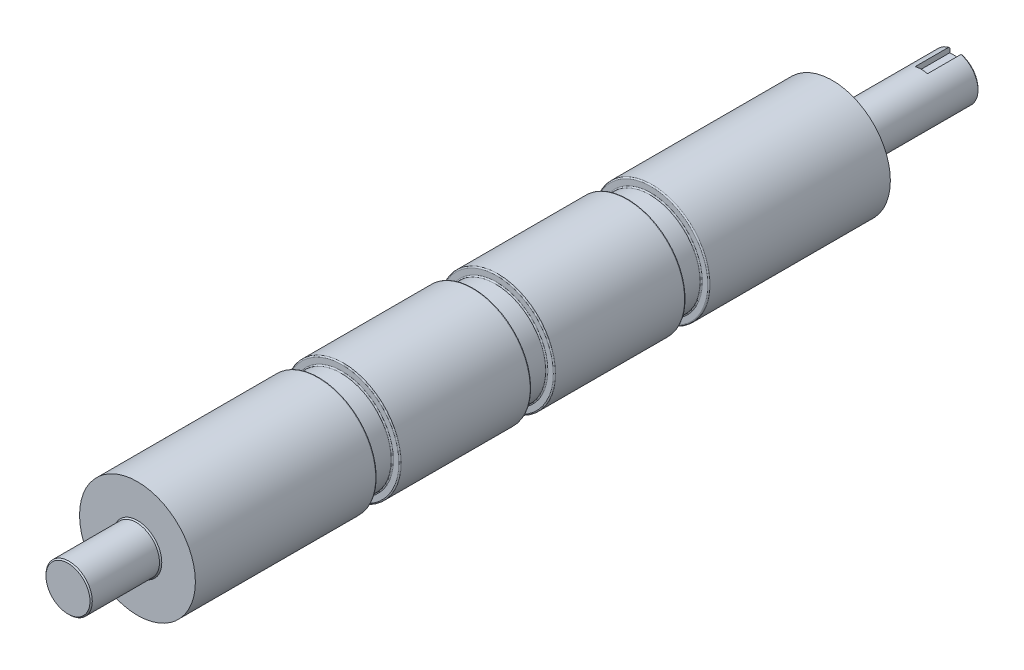
from build123d import *

# Parameters (mm, degrees)
SKETCH1_R                  = 150
BOSS_EXTRUDE1_DEPTH        = 1800
SKETCH2_W                  = 40
SKETCH2_H                  = 60
FILLET1_R                  = 3
LPATTERN1_COUNT            = 2
LPATTERN1_PITCH            = 400
FILLET1_OF_LPATTERN1_R     = 3
LPATTERN1_COL_COUNT        = 2
LPATTERN1_COL_PITCH        = 400
FILLET1_OF_LPATTERN1_COL_R = 3
SKETCH3_R                  = 60
BOSS_EXTRUDE2_DEPTH        = 180
CHAMFER1_SIZE              = 3
BOSS_EXTRUDE3_START        = 320
SKETCH4_R                  = 60
BOSS_EXTRUDE3_DEPTH        = 320
CHAMFER2_SIZE              = 3
SKETCH5_W                  = 32
SKETCH5_H                  = 32
CUT_EXTRUDE1_DEPTH         = 90


with BuildPart() as part:
    # Sketch1 → Boss-Extrude1 (new body)
    with BuildSketch(Plane.XY):
        Circle(SKETCH1_R)
    extrude(amount=BOSS_EXTRUDE1_DEPTH)

    # Sketch2 → Cut-Revolve1 (revolve, cut)
    with BuildSketch(Plane(origin=(0, 0, 0), x_dir=(1, 0, 0), z_dir=(0, 1, 0)), mode=Mode.PRIVATE) as cut_revolve1_sk:
        with Locations((150, -900)):
            Rectangle(SKETCH2_W, SKETCH2_H)
    cut_revolve1 = revolve(cut_revolve1_sk.sketch.rotate(Axis((0, 0, 0), (0, 0, 1)), 180), axis=Axis((0, 0, 0), (0, 0, 1)), mode=Mode.SUBTRACT)

    # Fillet1
    fillet1_edges = [part.edges().sort_by_distance(p)[0] for p in [
        (130, 0, 930),
        (-150, 0, 930),
        (130, 0, 870),
        (-150, 0, 870),
    ]]
    fillet(fillet1_edges, radius=FILLET1_R)

    # LPattern1: Cut-Revolve1 ×2
    with Locations(*[(0, 0, -i * LPATTERN1_PITCH) for i in range(1, LPATTERN1_COUNT)]):
        add(cut_revolve1, mode=Mode.SUBTRACT)

    # Fillet1 of LPattern1
    fillet1_of_lpattern1_edges = [part.edges().sort_by_distance(p)[0] for p in [
        (130, 0, 530),
        (-150, 0, 530),
        (130, 0, 470),
        (-150, 0, 470),
    ]]
    fillet(fillet1_of_lpattern1_edges, radius=FILLET1_OF_LPATTERN1_R)

    # LPattern1 col: Cut-Revolve1 ×2
    with Locations(*[(0, 0, i * LPATTERN1_COL_PITCH) for i in range(1, LPATTERN1_COL_COUNT)]):
        add(cut_revolve1, mode=Mode.SUBTRACT)

    # Fillet1 of LPattern1 col
    fillet1_of_lpattern1_col_edges = [part.edges().sort_by_distance(p)[0] for p in [
        (130, 0, 1330),
        (-150, 0, 1330),
        (130, 0, 1270),
        (-150, 0, 1270),
    ]]
    fillet(fillet1_of_lpattern1_col_edges, radius=FILLET1_OF_LPATTERN1_COL_R)

    # Sketch3 → Boss-Extrude2 (add)
    with BuildSketch(Plane.XY.offset(1800)):
        Circle(SKETCH3_R)
    extrude(amount=BOSS_EXTRUDE2_DEPTH)

    # Chamfer1
    chamfer1_edges = [part.edges().sort_by_distance(p)[0] for p in [
        (-60, 0, 1800),
        (-60, 0, 1980),
    ]]
    chamfer(chamfer1_edges, length=CHAMFER1_SIZE)

    # Sketch4 → Boss-Extrude3 (add)
    with BuildSketch(Plane(origin=(0, 0, 0), x_dir=(-1, 0, 0), z_dir=(0, 0, -1)).offset(BOSS_EXTRUDE3_START)):
        with Locations(Location((0, 0, 0), (0, 0, 180))):
            Circle(SKETCH4_R)
    extrude(amount=-BOSS_EXTRUDE3_DEPTH)

    # Chamfer2
    chamfer2_edges = [part.edges().sort_by_distance(p)[0] for p in [
        (-60, 0, 0),
        (-60, 0, -320),
    ]]
    chamfer(chamfer2_edges, length=CHAMFER2_SIZE)

    # Sketch5 → Cut-Extrude1 (cut)
    with BuildSketch(Plane(origin=(0, 0, -320), x_dir=(-1, 0, 0), z_dir=(0, 0, -1))):
        with Locations((0, 60)):
            Rectangle(SKETCH5_W, SKETCH5_H)
    extrude(amount=-CUT_EXTRUDE1_DEPTH, mode=Mode.SUBTRACT)


solid = part.part
